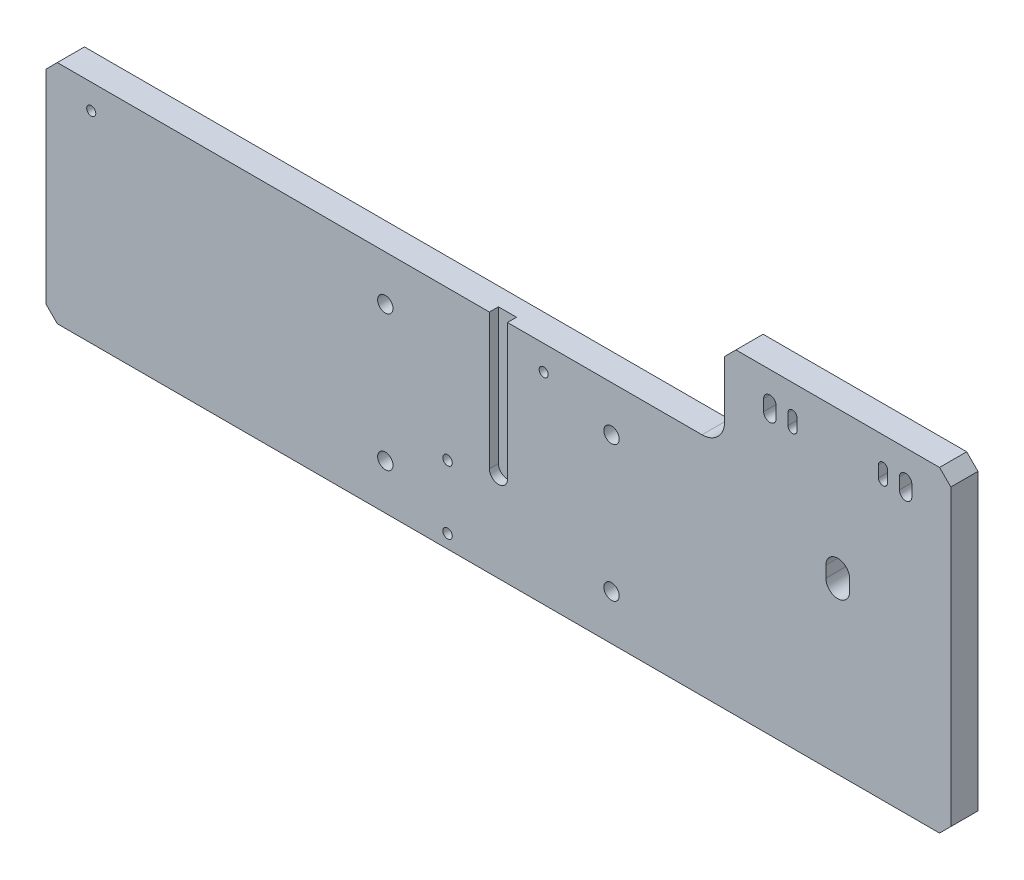
SolidWorks part; units mm, degrees
material "A6063"
ref_plane "Front Plane" through (0, 0, 0) normal (0, 0, 1) x (1, 0, 0)
ref_plane "Top Plane" through (0, 0, 0) normal (0, 1, 0) x (1, 0, 0)
ref_plane "Right Plane" through (0, 0, 0) normal (1, 0, 0) x (0, 0, -1)
sketch "Sketch1" plane through (0, 0, 0) normal (0, 0, 1) x (1, 0, 0)
  line L1 (-200, 50) -> (200, 50)
  line L2 (-200, 50) -> (-200, -50)
  line L3 (-200, -50) -> (200, -50)
  line L4 (200, 50) -> (200, -50)
  line L5 (-200, 50) -> (200, -50) construction
  line L6 (-200, -50) -> (200, 50) construction
  point P0 (0, 0)
  dimension "D1" = 400
  dimension "D2" = 100
extrude "Boss-Extrude1" add sketch "Sketch1" along normal blind 12
sketch "Sketch2" plane through (0, 50, 0) normal (0, 1, 0) x (1, 0, 0)
  line L0 (200, -12) -> (-200, -12) construction
  line L1 (200, 0) -> (100, 0)
  line L2 (200, 0) -> (200, -12)
  line L3 (200, -12) -> (100, -12)
  line L4 (100, 0) -> (100, -12)
  dimension "D1" = 100
extrude "Boss-Extrude2" add sketch "Sketch2" along normal blind 40
sketch "Sketch3" plane through (0, 0, 12) normal (0, 0, 1) x (1, 0, 0)
  line L0 (0, 0) -> (0, 50) construction
  line L1 (100, 50) -> (-200, 50) construction
  line L2 (0, 50) -> (0, -10) construction
  line L3 (4, 50) -> (4, -10)
  line L4 (-4, 50) -> (-4, -10)
  arc A0 (4, 50) -> (-4, 50) centre (0, 50) ccw
  arc A1 (-4, -10) -> (4, -10) centre (0, -10) ccw
  point P5 (0, 20)
  dimension "D2" = 60
  dimension "D1" = 8
extrude "Cut-Extrude1" cut sketch "Sketch3" against normal blind 4
hole_wizard "M8 Tapped Hole2" positions "Sketch5" profile "Sketch4" tap size "M8" standard "Iso"
sketch "Sketch5" plane through (0, -50, 0) normal (0, -1, 0) x (-1, 0, 0)
  line L0 (0, 0) -> (0, -12) construction
  line L1 (200, 0) -> (-200, 0) construction
  line L2 (200, -12) -> (-200, -12) construction
  point P0 (0, -6)
sketch "Sketch4" plane through (0, -50, 6) normal (1, 0, 0) x (0, 0, -1)
  line L0 (0, 0) -> (0, 24.0429)
  line L1 (0, 24.0429) -> (3.4, 22)
  line L2 (3.4, 22) -> (3.4, 0)
  line L5 (3.4, 0) -> (0, 0)
  line L10 (0, 24.0429) -> (-3.4, 22) construction
  line L11 (0, -6.35) -> (0, 107.95) construction
  dimension "螺纹孔钻头直径" = 6.8
  dimension "螺纹孔钻头深度" = 22
  dimension "导头角度" = 118
cosmetic thread "Hole thread1" parameters "D1"=18, "D2"=8
hole_wizard "M5 Tapped Hole1" positions "Sketch7" profile "Sketch6" tap size "M5" standard "Iso"
sketch "Sketch7" plane through (0, 0, 0) normal (0, 0, -1) x (-1, 0, 0)
  line L0 (200, -50) -> (-200, -50) construction
  line L1 (-200, -50) -> (-200, 90) construction
  point P0 (22.5, -16)
  point P3 (22.5, -44)
  dimension "D1" = 6
  dimension "D2" = 28
  dimension "D3" = 222.5
sketch "Sketch6" plane through (-22.5, -16, 0) normal (1, 0, 0) x (0, 1, 0)
  line L0 (0, 0) -> (0, 13.6618)
  line L1 (0, 13.6618) -> (2.1, 12.4)
  line L2 (2.1, 12.4) -> (2.1, 0)
  line L5 (2.1, 0) -> (0, 0)
  line L10 (0, 13.6618) -> (-2.1, 12.4) construction
  line L11 (0, -6.35) -> (0, 107.95) construction
  dimension "螺纹孔钻头直径" = 4.2
  dimension "螺纹孔钻头深度" = 12.4
  dimension "导头角度" = 118
cosmetic thread "Hole thread2" parameters "D1"=10, "D2"=5
cosmetic thread "Hole thread3" parameters "D1"=10, "D2"=5
hole_wizard "M4 Tapped Hole1" positions "Sketch9" profile "Sketch8" tap size "M4" standard "Iso"
sketch "Sketch9" plane through (0, 0, 0) normal (0, 0, -1) x (-1, 0, 0)
  line L0 (200, 50) -> (200, -50) construction
  line L1 (-100, 50) -> (200, 50) construction
  point P0 (180, 25)
  point P15 (140, 25)
  point P16 (100, 25)
  point P17 (60, 25)
  point P18 (20, 25)
  point P19 (-20, 25)
  dimension "D1" = 20
  dimension "D2" = 25
  dimension "D3" = 6
sketch "Sketch8" plane through (-180, 25, 0) normal (1, 0, 0) x (0, 1, 0)
  line L0 (0, 0) -> (0, 11.0914)
  line L1 (0, 11.0914) -> (1.65, 10.1)
  line L2 (1.65, 10.1) -> (1.65, 0)
  line L5 (1.65, 0) -> (0, 0)
  line L10 (0, 11.0914) -> (-1.65, 10.1) construction
  line L11 (0, -6.35) -> (0, 107.95) construction
  dimension "螺纹孔钻头直径" = 3.3
  dimension "螺纹孔钻头深度" = 10.1
  dimension "导头角度" = 118
cosmetic thread "Hole thread4" parameters "D1"=8, "D2"=4
cosmetic thread "Hole thread5" parameters "D1"=8, "D2"=4
cosmetic thread "Hole thread6" parameters "D1"=8, "D2"=4
cosmetic thread "Hole thread7" parameters "D1"=8, "D2"=4
cosmetic thread "Hole thread8" parameters "D1"=8, "D2"=4
cosmetic thread "Hole thread9" parameters "D1"=8, "D2"=4
sketch "Sketch10" plane through (0, 0, 0) normal (0, 0, -1) x (-1, 0, 0)
  line L0 (180, 25) -> (180, 42.831) construction
  line L1 (-100, 50) -> (200, 50) construction
  circle A0 centre (180, 39) radius 2
  circle A1 centre (-20, 39) radius 2
  dimension "D1" = 11
  dimension "D2" = 4
  dimension "D3" = 2
extrude "Cut-Extrude2" cut sketch "Sketch10" against normal through all
hole_wizard "M8 Tapped Hole1" positions "Sketch12" profile "Sketch11" tap size "M8" standard "Iso"
sketch "Sketch12" plane through (0, 0, 0) normal (0, 0, -1) x (-1, 0, 0)
  line L0 (0, 0) -> (0, -50) construction
  line L1 (200, -50) -> (-200, -50) construction
  line L3 (200, 0) -> (0, 0) construction
  line L4 (200, 50) -> (200, -50) construction
  point P0 (50, -30)
  point P2 (50, 30)
  point P16 (-50, -30)
  point P17 (-50, 30)
  dimension "D1" = 60
  dimension "D2" = 50
sketch "Sketch11" plane through (-50, -30, 0) normal (1, 0, 0) x (0, 1, 0)
  line L0 (0, 0) -> (0, 21.7929)
  line L1 (0, 21.7929) -> (3.4, 19.75)
  line L2 (3.4, 19.75) -> (3.4, 0)
  line L5 (3.4, 0) -> (0, 0)
  line L10 (0, 21.7929) -> (-3.4, 19.75) construction
  line L11 (0, -6.35) -> (0, 107.95) construction
  dimension "螺纹孔钻头直径" = 6.8
  dimension "螺纹孔钻头深度" = 19.75
  dimension "导头角度" = 118
cosmetic thread "Hole thread10" parameters "D1"=12, "D2"=8
cosmetic thread "Hole thread11" parameters "D1"=12, "D2"=8
cosmetic thread "Hole thread12" parameters "D1"=12, "D2"=8
cosmetic thread "Hole thread13" parameters "D1"=12, "D2"=8
hole_wizard "Ø5.5 (5.5) Diameter Hole1" positions "Sketch14" profile "Sketch13" hole size "Ø5.5" standard "Iso"
sketch "Sketch14" plane through (0, 0, 12) normal (0, 0, 1) x (1, 0, 0)
  line L0 (150, 90) -> (150, 34.915) construction
  line L1 (100, 90) -> (200, 90) construction
  point P0 (120, 75)
  point P3 (180, 75)
  point P6 (150, 25)
  dimension "D1" = 60
  dimension "D2" = 15
  dimension "D3" = 50
sketch "Sketch13" plane through (120, 75, 12) normal (1, 0, 0) x (0, -1, 0)
  line L0 (0, 0) -> (0, 77.6524)
  line L1 (0, 77.6524) -> (2.75, 76)
  line L2 (2.75, 76) -> (2.75, 0)
  line L5 (2.75, 0) -> (0, 0)
  line L10 (0, 77.6524) -> (-2.75, 76) construction
  line L11 (0, -6.35) -> (0, 107.95) construction
  dimension "孔直径" = 5.5
  dimension "孔深度" = 76
  dimension "导头角度" = 118
sketch "Sketch15" plane through (0, 0, 12) normal (0, 0, 1) x (1, 0, 0)
  line L0 (120, 77.5) -> (120, 72.5) construction
  line L1 (122.75, 77.5) -> (122.75, 72.5)
  line L2 (117.25, 77.5) -> (117.25, 72.5)
  line L3 (180, 77.5) -> (180, 72.5) construction
  line L4 (182.75, 77.5) -> (182.75, 72.5)
  line L5 (177.25, 77.5) -> (177.25, 72.5)
  line L6 (150, 27.5) -> (150, 22.5) construction
  line L7 (155.25, 27.5) -> (155.25, 22.5)
  line L8 (144.75, 27.5) -> (144.75, 22.5)
  arc A0 (122.75, 77.5) -> (117.25, 77.5) centre (120, 77.5) ccw
  arc A1 (117.25, 72.5) -> (122.75, 72.5) centre (120, 72.5) ccw
  arc A2 (182.75, 77.5) -> (177.25, 77.5) centre (180, 77.5) ccw
  arc A3 (177.25, 72.5) -> (182.75, 72.5) centre (180, 72.5) ccw
  arc A4 (155.25, 27.5) -> (144.75, 27.5) centre (150, 27.5) ccw
  arc A5 (144.75, 22.5) -> (155.25, 22.5) centre (150, 22.5) ccw
  point P2 (120, 75)
  point P9 (180, 75)
  point P17 (150, 25)
  dimension "D1" = 5
  dimension "D2" = 10.5
  dimension "D3" = 5.5
  dimension "D4" = 5
extrude "Cut-Extrude3" cut sketch "Sketch15" against normal through all
chamfer "Chamfer1" distance 5 angle 45 5 edges at (100, 90, 6) (200, 90, 6) (200, -50, 6) (-200, 50, 6) (-200, -50, 6)
fillet "Fillet1" radius 10 1 edges
sketch "Sketch16" plane through (0, 0, 0) normal (0, 0, -1) x (-1, 0, 0)
  line L0 (-120, 72.5) -> (-180, 72.5) construction
  line L1 (-120, 77.5) -> (-180, 77.5) construction
  line L2 (-130, 72.5) -> (-130, 77.5) construction
  line L3 (-132, 72.5) -> (-132, 77.5)
  line L4 (-128, 72.5) -> (-128, 77.5)
  line L5 (-170, 72.5) -> (-170, 77.5) construction
  line L6 (-172, 72.5) -> (-172, 77.5)
  line L7 (-168, 72.5) -> (-168, 77.5)
  arc A0 (-132, 72.5) -> (-128, 72.5) centre (-130, 72.5) ccw
  arc A1 (-128, 77.5) -> (-132, 77.5) centre (-130, 77.5) ccw
  arc A2 (-172, 72.5) -> (-168, 72.5) centre (-170, 72.5) ccw
  arc A3 (-168, 77.5) -> (-172, 77.5) centre (-170, 77.5) ccw
  point P10 (-130, 75)
  point P15 (-170, 75)
  dimension "D1" = 4
  dimension "D2" = 4
  dimension "D3" = 10
  dimension "D4" = 10
extrude "Cut-Extrude4" cut sketch "Sketch16" against normal through all
